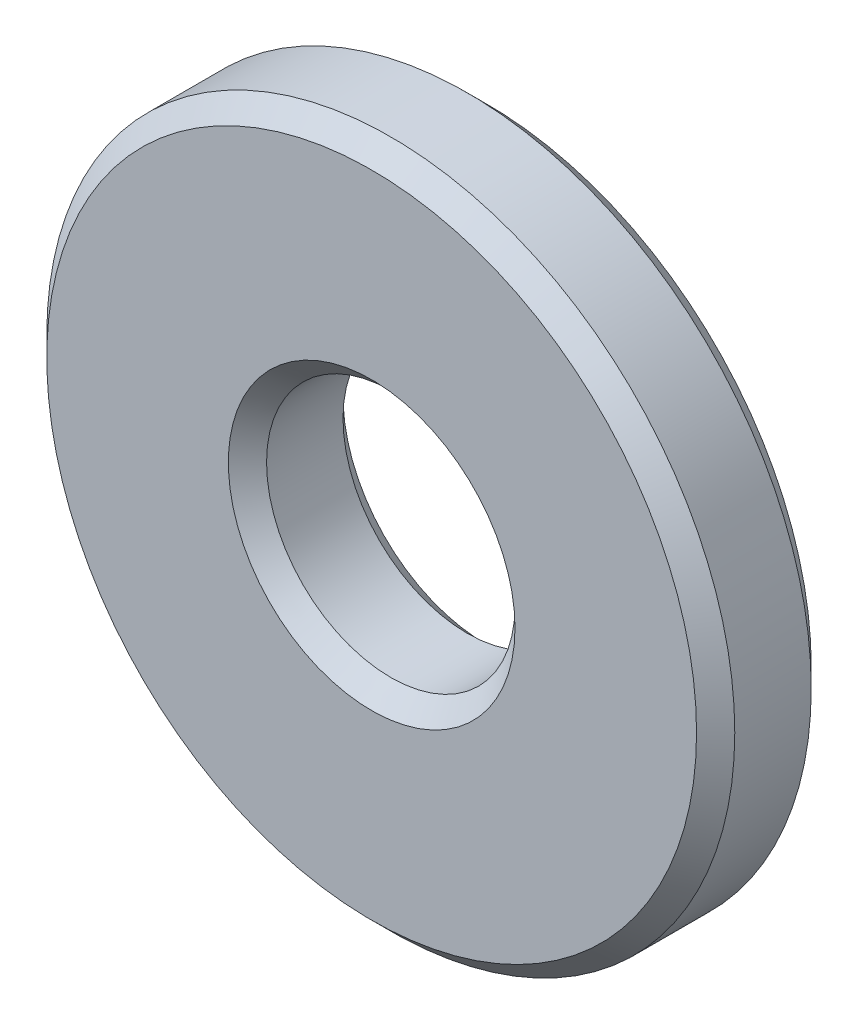
SolidWorks part; units mm, degrees
ref_plane "Front Plane" through (0, 0, 0) normal (0, 0, 1) x (1, 0, 0)
ref_plane "Top Plane" through (0, 0, 0) normal (0, 1, 0) x (1, 0, 0)
ref_plane "Right Plane" through (0, 0, 0) normal (1, 0, 0) x (0, 0, -1)
sketch "Sketch1" plane through (0, 0, 0) normal (0, 0, 1) x (1, 0, 0)
  circle A0 centre (0, 0) radius 3.25
  circle A1 centre (0, 0) radius 9
  dimension "D1" = 6.5
  dimension "D2" = 18
extrude "Boss-Extrude1" add sketch "Sketch1" along normal blind 3
chamfer "Chamfer1" distance 0.5 angle 45 4 edges at (9, 0, 0) (9, 0, 3) (3.25, 0, 0) (3.25, 0, 3)
